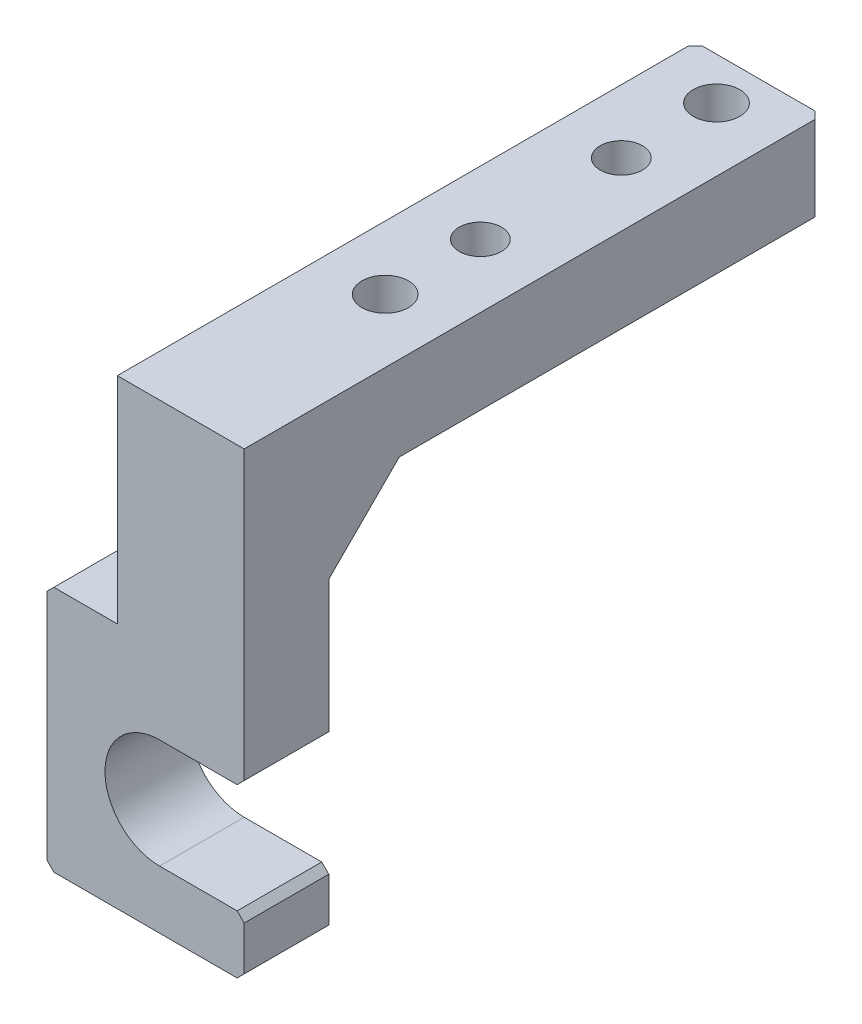
SolidWorks part; units mm, degrees
material "#45(1.1191)"
ref_plane "前视基准面" through (0, 0, 0) normal (0, 0, 1) x (1, 0, 0)
ref_plane "上视基准面" through (0, 0, 0) normal (0, 1, 0) x (1, 0, 0)
ref_plane "右视基准面" through (0, 0, 0) normal (1, 0, 0) x (0, 0, -1)
sketch "草图1" plane through (0, 0, 0) normal (0, 0, 1) x (1, 0, 0)
  line L1 (-9, -32.75) -> (9, -32.75)
  line L2 (-9, -32.75) -> (-9, 32.75)
  line L3 (-9, 32.75) -> (9, 32.75)
  line L4 (9, -32.75) -> (9, 32.75)
  line L5 (-9, -32.75) -> (9, 32.75) construction
  line L6 (-9, 32.75) -> (9, -32.75) construction
  point P0 (0, 0)
  dimension "D1" = 18
  dimension "D2" = 65.5
extrude "凸台-拉伸1" add sketch "草图1" along normal mid plane 12
sketch "草图2" plane through (0, 0, 6) normal (0, 0, 1) x (1, 0, 0)
  line L0 (-9, -32.75) -> (9, -32.75) construction
  line L1 (-19, 2.25) -> (9, 2.25)
  line L2 (-19, 2.25) -> (-19, -32.75)
  line L3 (-19, -32.75) -> (9, -32.75)
  line L4 (9, 2.25) -> (9, -32.75)
  line L5 (-19, 2.25) -> (9, -32.75) construction
  line L6 (-19, -32.75) -> (9, 2.25) construction
  line L7 (9, -32.75) -> (9, 32.75) construction
  point P0 (-5, -15.25)
  dimension "D1" = 28
  dimension "D2" = 35
extrude "凸台-拉伸2" add sketch "草图2" against normal up to surface (12 mm away) up to face at (0, 0, -6)
sketch "草图3" plane through (0, 0, 6) normal (0, 0, 1) x (1, 0, 0)
  line L0 (-3, -16.75) -> (21, -16.75) construction
  line L2 (-3, -9) -> (21, -9)
  line L3 (-3, -24.5) -> (21, -24.5)
  line L4 (9, 32.75) -> (-9, 32.75) construction
  line L5 (9, -32.75) -> (9, 32.75) construction
  line L7 (9, -32.75) -> (9, 32.75) construction
  arc A0 (-3, -9) -> (-3, -24.5) centre (-3, -16.75) ccw
  arc A1 (21, -24.5) -> (21, -9) centre (21, -16.75) ccw
  point P4 (9, -16.75)
  dimension "D1" = 15.5
  dimension "D2" = 49.5
  dimension "D3" = 12
extrude "切除-拉伸1" cut sketch "草图3" against normal through all
sketch "草图4" plane through (0, 0, -6) normal (0, 0, -1) x (-1, 0, 0)
  line L0 (-9, -9) -> (-9, 32.75) construction
  line L1 (9, 32.75) -> (-9, 32.75)
  line L2 (9, 32.75) -> (9, 20.75)
  line L3 (9, 20.75) -> (-9, 20.75)
  line L4 (-9, 32.75) -> (-9, 20.75)
  dimension "D1" = 12
extrude "凸台-拉伸3" add sketch "草图4" along normal blind 70
chamfer "倒角1" distance 10 angle 45 1 edges at (0, 20.75, -6)
sketch "草图5" plane through (0, 20.75, 0) normal (0, -1, 0) x (-1, 0, 0)
  line L0 (0, 23) -> (0, 70) construction
  line L1 (0, 70) -> (0, 76) construction
  line L2 (-9, 76) -> (9, 76) construction
  point P0 (0, 23)
  point P2 (0, 70)
  dimension "D1" = 6
  dimension "D2" = 47
hole_wizard "M6 六角凹头螺钉的柱形沉头孔1" positions "草图5" profile "草图6" counterbore size "M6" standard "ISO" end condition through all
sketch "草图6" plane through (0, 20.75, -23) normal (1, 0, 0) x (0, 0, -1)
  line L0 (0, 0) -> (0, 12)
  line L1 (0, 12) -> (3.3, 12)
  line L3 (3.3, 12) -> (3.3, 6.4)
  line L4 (3.3, 6.4) -> (5.5, 6.4)
  line L5 (5.5, 6.4) -> (5.5, 0)
  line L7 (5.5, 0) -> (0, 0)
  line L11 (0, -6.35) -> (0, 107.95) construction
  dimension "通孔孔直径" = 6.6
  dimension "通孔孔深度" = 12
  dimension "柱形沉头孔直径" = 11
  dimension "柱形沉头孔深度" = 6.4
sketch "草图7" plane through (0, 20.75, 0) normal (0, -1, 0) x (-1, 0, 0)
  line L0 (0, 23) -> (0, 36.5) construction
  line L1 (0, 36.5) -> (0, 56.5) construction
  line L2 (0, 56.5) -> (0, 70) construction
  point P0 (0, 36.5)
  point P2 (0, 56.5)
  dimension "D1" = 20
hole_wizard "Ø6.0mm 暗销孔1" positions "草图7" profile "草图8" hole size "Ø6.0" standard "ISO" end condition through all
sketch "草图8" plane through (0, 20.75, -36.5) normal (1, 0, 0) x (0, 0, -1)
  line L0 (0, 0) -> (0, 12)
  line L1 (0, 12) -> (3, 12)
  line L2 (3, 12) -> (3, 0)
  line L5 (3, 0) -> (0, 0)
  line L11 (0, -6.35) -> (0, 107.95) construction
  dimension "通孔孔直径" = 6
  dimension "通孔孔深度" = 12
chamfer "倒角2" distance 1 angle 45 7 edges at (9, -24.5, 0) (9, -9, 0) (-19, 2.25, 0) (-19, -32.75, 0) (9, -32.75, 0) (-9, 26.75, -76) (9, 26.75, -76)
